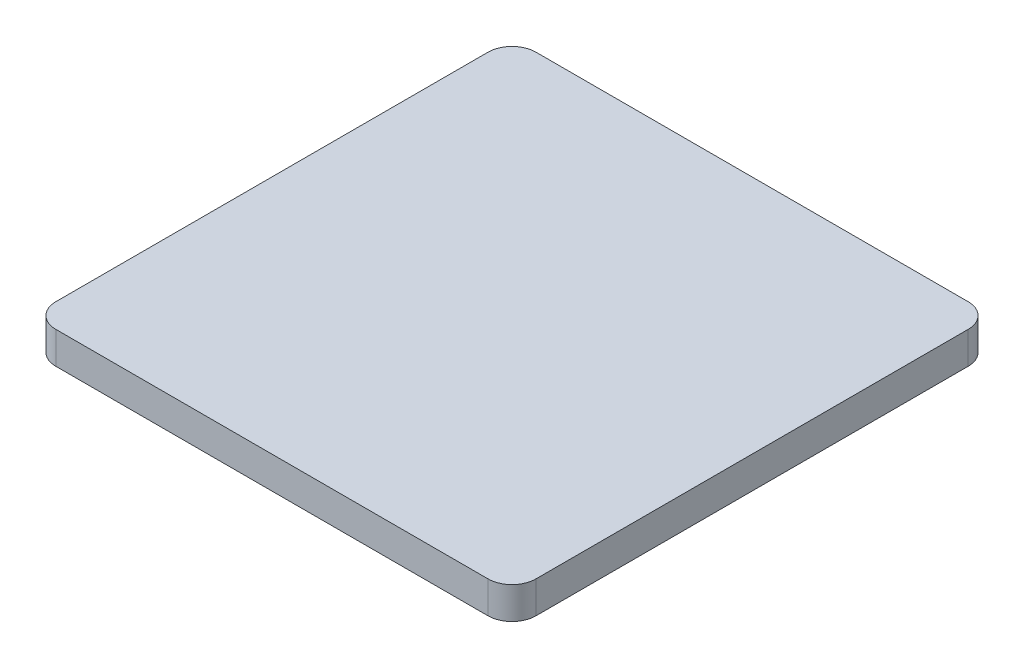
SolidWorks part; units mm, degrees
ref_plane "Front Plane" through (0, 0, 0) normal (0, 0, 1) x (1, 0, 0)
ref_plane "Top Plane" through (0, 0, 0) normal (0, 1, 0) x (1, 0, 0)
ref_plane "Right Plane" through (0, 0, 0) normal (1, 0, 0) x (0, 0, -1)
sketch "Sketch 1" plane through (0, 0, 0) normal (0, 1, 0) x (1, 0, 0)
  line L0 (0, 129.8246) -> (0, -147.3684) construction
  line L1 (-161.4035, 0) -> (194.7368, 0) construction
  line L2 (135, 150) -> (-135, 150)
  line L3 (-150, 135) -> (-150, -135)
  line L4 (135, -150) -> (-135, -150)
  line L5 (150, 135) -> (150, -135)
  circle A0 centre (-90, 90) radius 15 construction
  arc A1 (-135, 150) -> (-150, 135) centre (-135, 135) ccw
  arc A2 (-135, -150) -> (-150, -135) centre (-135, -135) cw
  arc A3 (135, -150) -> (150, -135) centre (135, -135) ccw
  arc A4 (135, 150) -> (150, 135) centre (135, 135) cw
  point P7 (150, 0)
  point P9 (0, 150)
  point P15 (-150, 0)
  point P22 (0, -150)
  dimension "D3" = 30
  dimension "D4" = 15
  dimension "D5" = 60
  dimension "D6" = 60
  dimension "D1" = 300
  dimension "D2" = 300
extrude "Boss-Extrude 1" add sketch "Sketch 1" along normal blind 20
